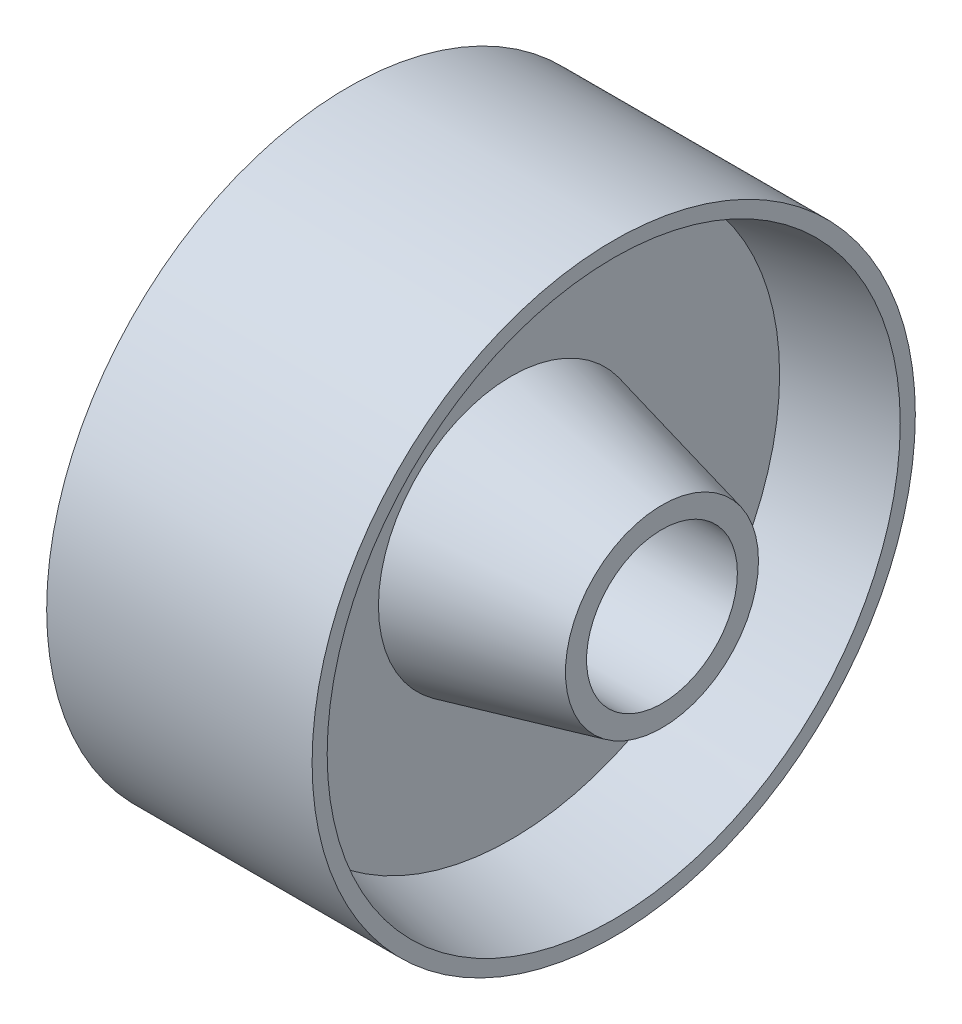
from build123d import *


with BuildPart() as part:
    # Sketch1 → Revolve1 (revolve)
    with BuildSketch(Plane.XY, mode=Mode.PRIVATE) as revolve1_sk:
        Polygon((-762, 317.5), (-762, 406.4), (-127, 558.8), (-127, 1130.3), (-558.8, 1206.5), (-558.8, 1270), (558.8, 1270), (558.8, 1206.5), (127, 1130.3), (127, 558.8), (762, 406.4), (762, 317.5), align=None)
    revolve(revolve1_sk.sketch.rotate(Axis((0, 0, 0), (-1, 0, 0)), 90), axis=Axis((0, 0, 0), (-1, 0, 0)))


solid = part.part
